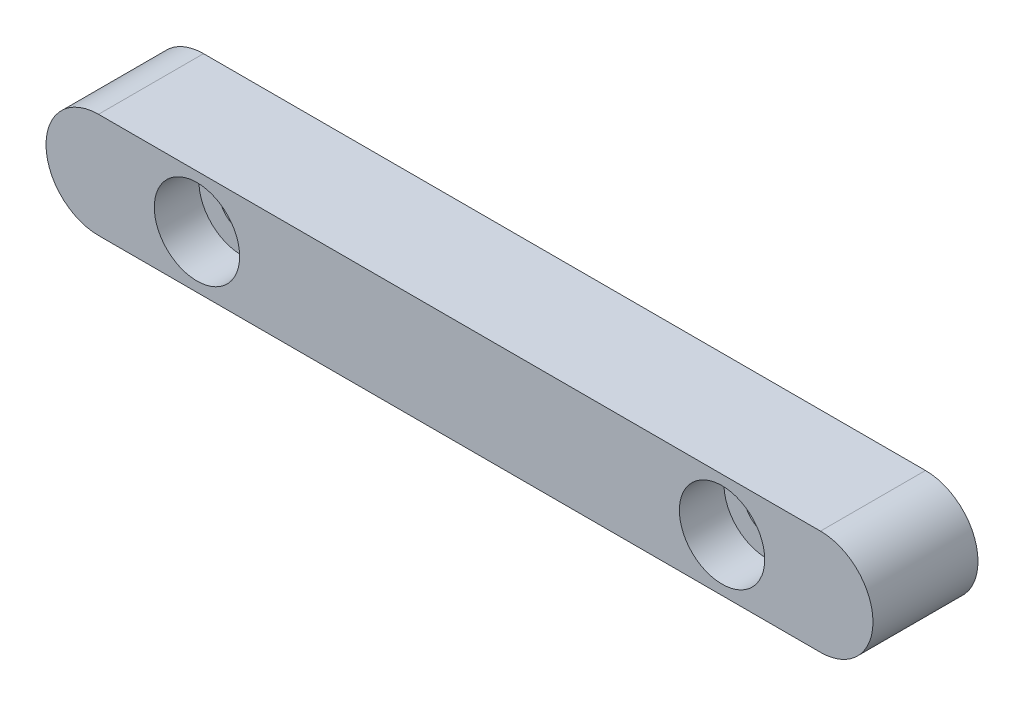
from build123d import *

# Parameters (mm, degrees)
BOSS_EXTRUDE1_DEPTH                                 = 8
CBORE_FOR_M3_HEX_SOCKET_HEAD_CAP_SCREW1_D           = 3.4
CBORE_FOR_M3_HEX_SOCKET_HEAD_CAP_SCREW1_CBORE_D     = 6.5
CBORE_FOR_M3_HEX_SOCKET_HEAD_CAP_SCREW1_CBORE_DEPTH = 3.4


with BuildPart() as part:
    # Sketch1 → Boss-Extrude1 (new body)
    with BuildSketch(Plane.XY):
        with BuildLine():
            Line((-27.5, 4), (27.5, 4))
            ThreePointArc((27.5, 4), (31.5, 0), (27.5, -4))
            Line((27.5, -4), (-27.5, -4))
            ThreePointArc((-27.5, -4), (-31.5, 0), (-27.5, 4))
        make_face()
    extrude(amount=BOSS_EXTRUDE1_DEPTH)

    # CBORE for M3 Hex Socket Head Cap Screw1 (through all)
    with Locations(Plane.XY.offset(8)):
        with Locations((-20, 0), (20, 0)):
            CounterBoreHole(CBORE_FOR_M3_HEX_SOCKET_HEAD_CAP_SCREW1_D / 2, CBORE_FOR_M3_HEX_SOCKET_HEAD_CAP_SCREW1_CBORE_D / 2, CBORE_FOR_M3_HEX_SOCKET_HEAD_CAP_SCREW1_CBORE_DEPTH)


solid = part.part
